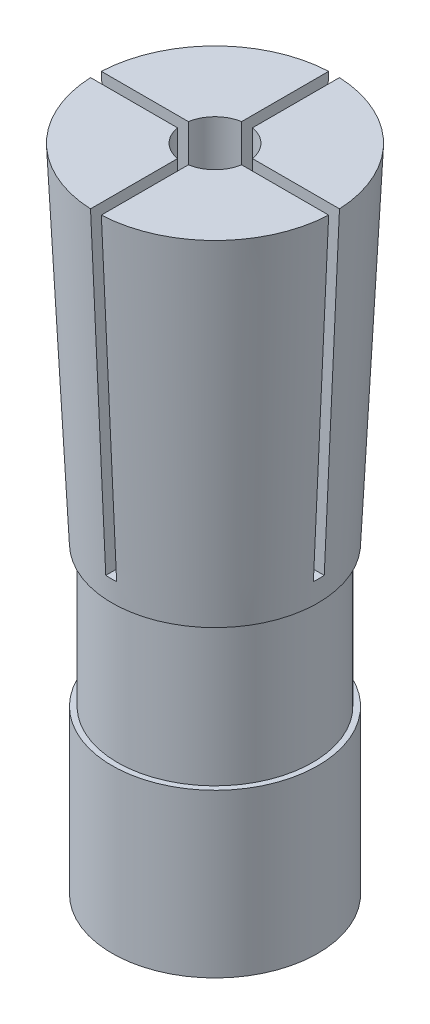
from build123d import *

# Parameters (mm, degrees)
SKETCH_2_R              = 3
CUT_EXTRUDE_1_DEPTH     = 62.983868869
HOLE_WIZARD_M10_1_D     = 8.5
HOLE_WIZARD_M10_1_DEPTH = 24.5
HOLE_WIZARD_M10_1_TIP   = 2.553657631
SKETCH_4_W              = 50
SKETCH_4_H              = 1
CUT_EXTRUDE_2_DEPTH     = 30
SKETCH_5_W              = 1
SKETCH_5_H              = 50
CUT_EXTRUDE_3_DEPTH     = 30


with BuildPart() as part:
    # 草图1 → 旋转1 (revolve)
    with BuildSketch(Plane.XY, mode=Mode.PRIVATE) as revolve_1_sk:
        Polygon((0, 60), (11, 60), (9.5, 28), (9, 28), (9, 15), (9.5, 15), (9.5, 0), (0, 0), align=None)
    revolve(revolve_1_sk.sketch.rotate(Axis((0, 0, 0), (0, 1, 0)), 90), axis=Axis((0, 0, 0), (0, 1, 0)))

    # 草图2 → 切除-拉伸1 (cut, through all)
    with BuildSketch(Plane(origin=(0, 60, 0), x_dir=(1, 0, 0), z_dir=(0, 1, 0))):
        with Locations(Location((0, 0, 0), (0, 0, 270))):
            Circle(SKETCH_2_R)
    extrude(amount=-CUT_EXTRUDE_1_DEPTH, mode=Mode.SUBTRACT)

    # M10 螺纹孔1
    with Locations(Plane(origin=(0, 0, 0), x_dir=(0, 0, -1), z_dir=(0, -1, 0))):
        with Locations((0, 0)):
            Hole(HOLE_WIZARD_M10_1_D / 2, depth=HOLE_WIZARD_M10_1_DEPTH)
            with Locations((0, 0, -(HOLE_WIZARD_M10_1_DEPTH + HOLE_WIZARD_M10_1_TIP / 2))):  # 118° drill point
                Cone(0, HOLE_WIZARD_M10_1_D / 2, HOLE_WIZARD_M10_1_TIP, mode=Mode.SUBTRACT)

    # 草图4 → 切除-拉伸2 (cut)
    with BuildSketch(Plane(origin=(0, 60, 0), x_dir=(1, 0, 0), z_dir=(0, 1, 0))):
        Rectangle(SKETCH_4_W, SKETCH_4_H)
    extrude(amount=-CUT_EXTRUDE_2_DEPTH, mode=Mode.SUBTRACT)

    # 草图5 → 切除-拉伸3 (cut)
    with BuildSketch(Plane(origin=(0, 60, 0), x_dir=(1, 0, 0), z_dir=(0, 1, 0))):
        Rectangle(SKETCH_5_W, SKETCH_5_H)
    extrude(amount=-CUT_EXTRUDE_3_DEPTH, mode=Mode.SUBTRACT)


solid = part.part
